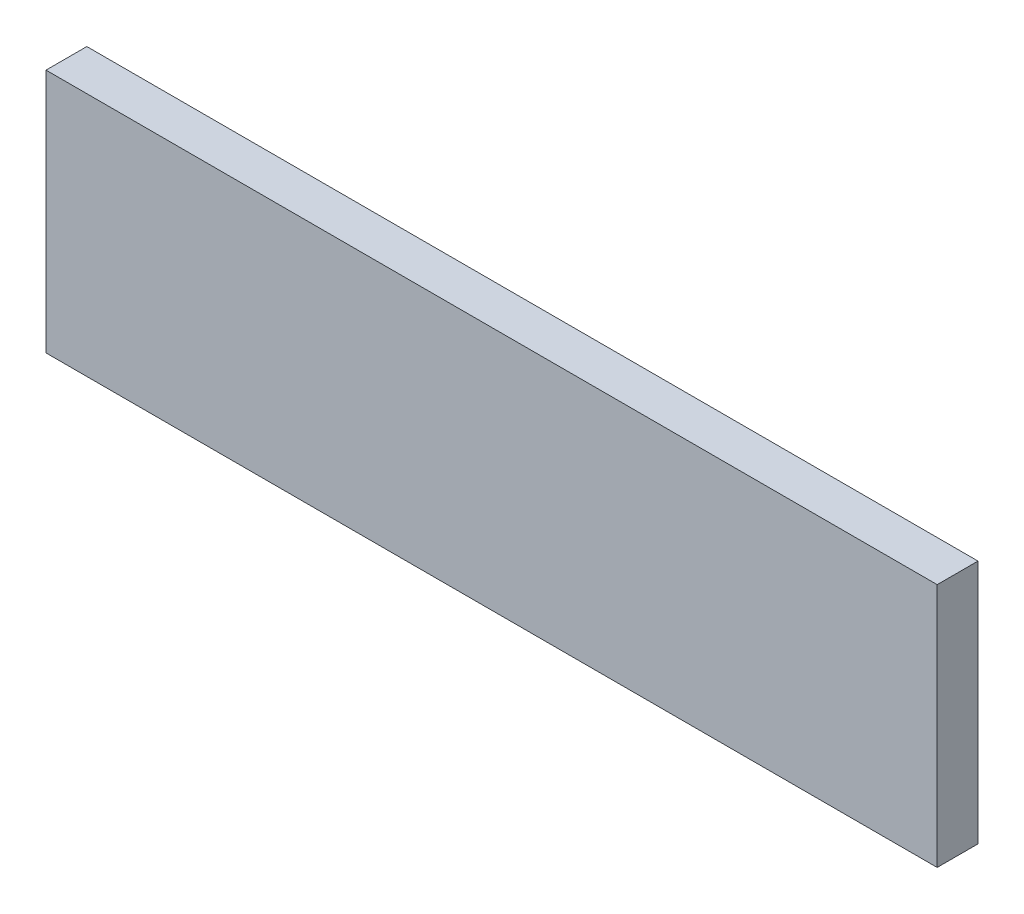
from build123d import *

# Parameters (mm, degrees)
SKETCH_1_W      = 218.3
SKETCH_1_H      = 60
EXTRUDE_1_DEPTH = 10


with BuildPart() as part:
    # 草图1 → 凸台-拉伸1 (new body)
    with BuildSketch(Plane.XY):
        Rectangle(SKETCH_1_W, SKETCH_1_H)
    extrude(amount=EXTRUDE_1_DEPTH)


solid = part.part
